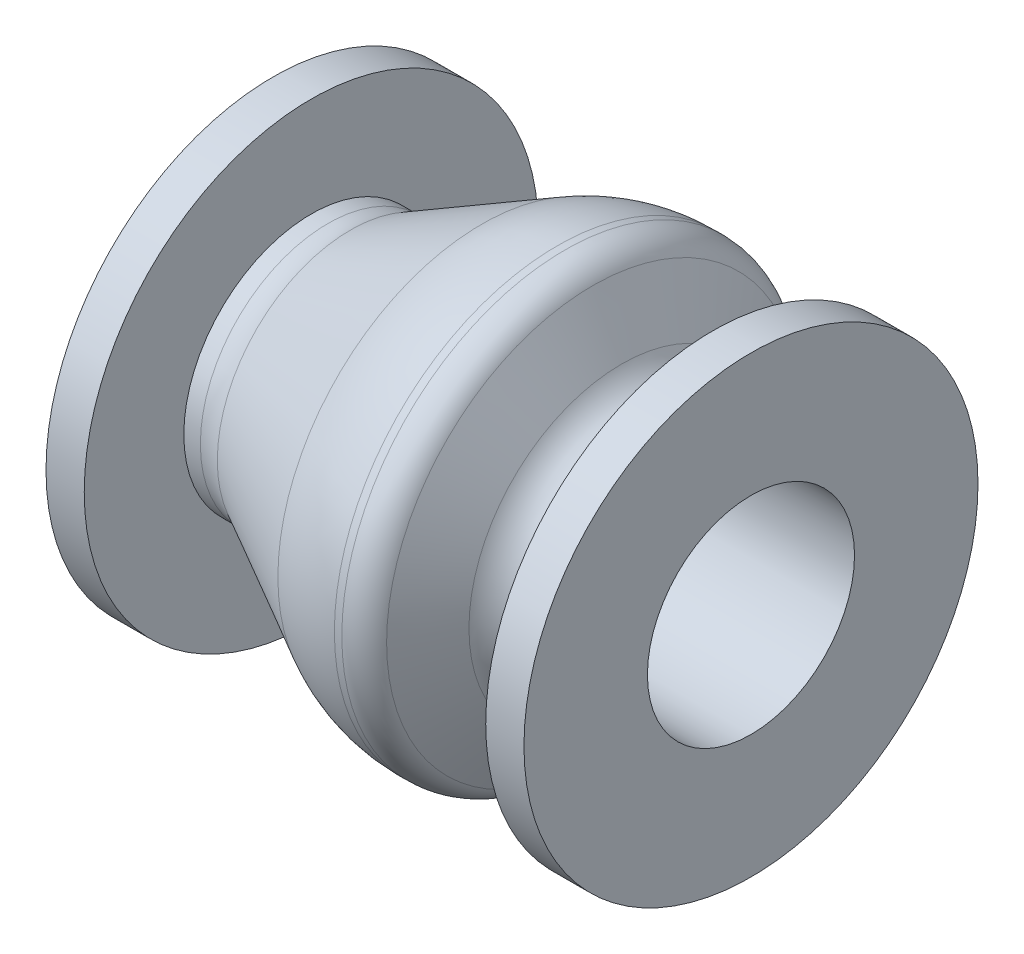
from build123d import *


with BuildPart() as part:
    # Sketch1 → Revolve1 (revolve)
    with BuildSketch(Plane.XY, mode=Mode.PRIVATE) as revolve1_sk:
        with BuildLine():
            Line((0, 65), (0, 142.5))
            Line((0, 142.5), (24, 142.5))
            Line((24, 142.5), (24, 80))
            Line((24, 80), (34.398449785, 80))
            ThreePointArc((34.398449785, 80), (41.732480398, 80.910276815), (48.621444476, 83.585867002))
            Line((48.621444476, 83.585867002), (130.980482924, 127.933041551))
            ThreePointArc((130.980482924, 127.933041551), (153.943696517, 136.851675508), (178.390465228, 139.885931559))
            Line((178.390465228, 139.885931559), (183.05792065, 139.885931559))
            ThreePointArc((183.05792065, 139.885931559), (193.313652481, 137.056253763), (200.667342649, 129.36792802))
            Line((200.667342649, 129.36792802), (218.75476257, 95.777005309))
            ThreePointArc((218.75476257, 95.777005309), (229.785297821, 84.244516693), (245.168895567, 80))
            Line((245.168895567, 80), (276, 80))
            Line((276, 80), (276, 142.5))
            Line((276, 142.5), (300, 142.5))
            Line((300, 142.5), (300, 65))
            Line((300, 65), (0, 65))
        make_face()
    revolve(revolve1_sk.sketch.rotate(Axis((0, 0, 0), (1, 0, 0)), 90), axis=Axis((0, 0, 0), (1, 0, 0)))


solid = part.part
